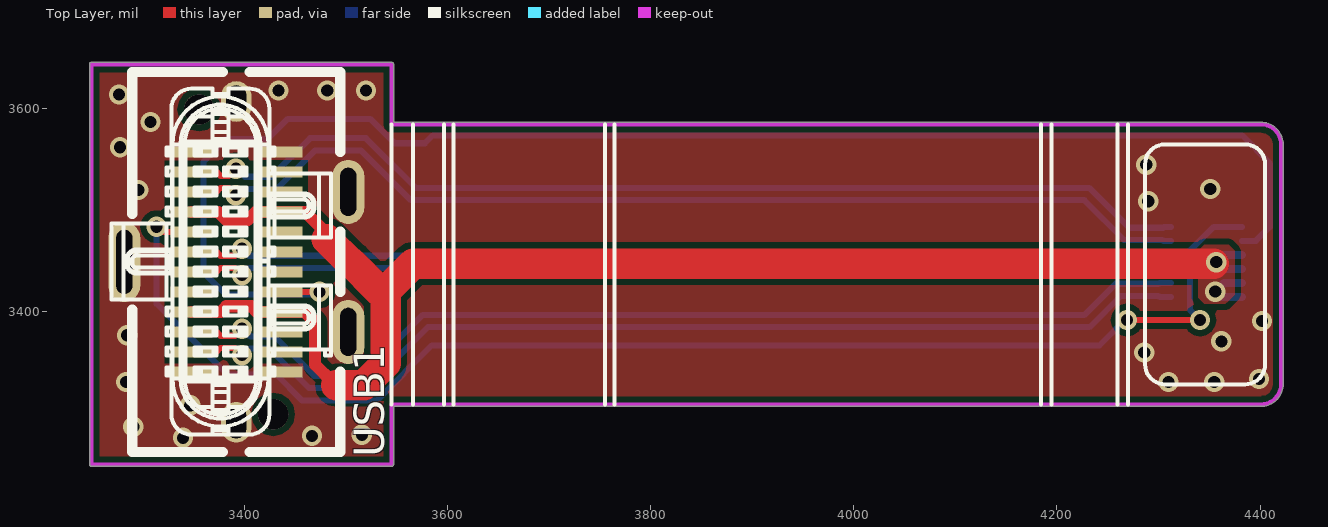
[diagram p0: Top Layer view]
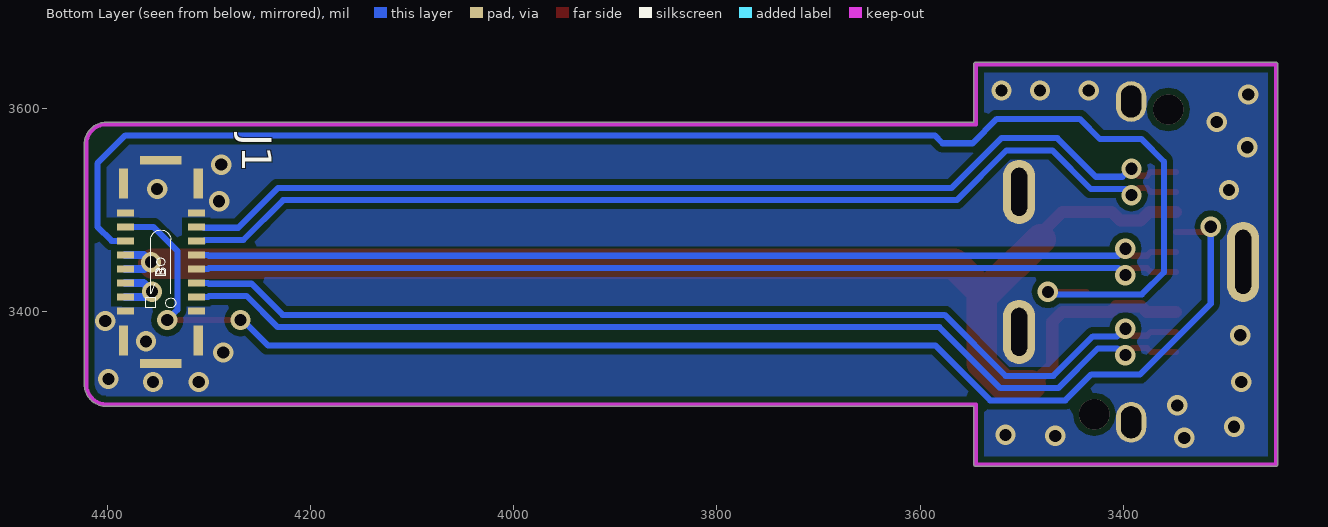
[diagram p1: Bottom Layer view, seen from below]
# Altium PCB MISC89352.pcbdoc
Units mil, origin at the board's own origin, x right, y up, seen from the top; angles counter-clockwise.
Board outline 1174.69 x 397.67 mil, 2 copper layers (Top Layer, Bottom Layer); 2 components, 10 nets, 53 pads, 35 vias.

## Layer stack, top to bottom (the 12.6 mil dielectric is the usual default, probably not edited)
Top Layer: signal copper 1.4
Dielectric: dielectric 12.6, FR-4, Dk 4.8
Bottom Layer: signal copper 1.4

## Board outline
3250,3248.02 cw(c3250,3250) 3248.02,3250 3248.02,3643.7 cw(c3250,3643.7) 3250,3645.68 3545.28,3645.68 cw(c3545.28,3643.7) 3547.26,3643.7 3547.26,3586.63 4401.04,3586.63 cw(c4401.04,3564.96) 4422.7,3564.96 4422.7,3328.74 cw(c4401.04,3328.74) 4401.04,3307.07 3547.26,3307.07 3547.26,3250 cw(c3545.28,3250) 3545.28,3248.02

## Design rules (kind name [scope] priority, off if disabled: settings)
Clearance [All] p1: gap=6
DiffPairsRouting [All] p1: maxlimit=6 minlimit=6 mostfreqgap=6 maxuncoupledlength=500
HoleSize [All] p1: absolutevalues=TRUE maxlimit=500 minlimit=1 maxpercent=80.000 minpercent=20.000
HoleToHoleClearance [All] p1: gap=0 allowstackedmicrovias=TRUE
MinimumSolderMaskSliver [All] p1: minsoldermaskwidth=0
PlaneConnect [All] p1: planeconnectstyle=Direct reliefexpansion=20 reliefentries=4 reliefconductorwidth=10 reliefairgap=10
PolygonConnect [All] p1: connectstyle=Direct reliefconductorwidth=10 reliefentries=4 polygonreliefangle="90 Angle"
RoutingVias [All] p1: holewidth=12 width=20 viastyle="Through Hole" minholewidth=12 minwidth=20 maxholewidth=12 maxwidth=20
SilkToSilkClearance [All] p1: silktosilkclearance=0
SilkscreenOverComponentPads [All] p1: minsilkscreentomaskgap=0
SolderMaskExpansion [All] p1: expansion=4
Width [All] p1: maxlimit=40 minlimit=6 preferedwidth=6 minimp=50.000000 maximp=50.000000 favimp=50.000000
21 further rules are at their usual default settings.

## Classes and differential pairs
differential pair D_D2: +DP2 -DN2
differential pair D_RX1: +RXP1 -RXN1
differential pair D_TX2: +TXP2 -TXN2

## Components (designator, comment, footprint, x,y, rotation, side; value= is the part's Value field where it differs from the comment)
J1 "BK13C06-16DS" BK13C06-16DS_AA 4347.41,3449.24 r90 bottom
USB1 "TYPEC-952-ACP24" USB-C-SMD_TYPEC-952-ACP24 3392.41,3449.24 r270 top locked

## Footprints (in the part's own frame and the unit in brackets; to place one, negate y for a bottom-side part, rotate by r counter-clockwise, add the part's x,y. Pads: shape width x height; smd on the part's side, far side on the other; paste and mask are expansions set on the pad)
BK13C06-16DS_AA [mm]
  rect 0.18x0.425 smd paste+0.102 mask+0.072: 1(-1.225,-0.887) 2(-0.875,-0.887) 3(-0.525,-0.887) 4(-0.175,-0.887) 5(0.175,-0.887) 6(0.525,-0.887) 7(0.875,-0.887) 8(1.225,-0.887) 9(1.225,0.887) 10(0.875,0.887) 11(0.525,0.887) 12(0.175,0.887) 13(-0.175,0.887) 14(-0.525,0.887) 15(-0.875,0.887) 16(-1.225,0.887)
  rect 0.75x0.235 smd paste+0.102 mask+0.05: 17(-1.96,0.932) 18(-1.96,-0.932) 20(1.96,0.932) 21(1.96,-0.932)
  rect 0.215x1.04 smd paste+0.102 mask+0.05: 19(-2.54,0) 22(2.54,0)
  silkscreen extent -1.15,-0.37 0.8,0.38
USB-C-SMD_TYPEC-952-ACP24 [mm]
  round 0.76 hole 0.76 unplated: 0(-3.81,-0.93) 0(3.81,0.92)
  oval 1.6x0.8 hole 0.4 slot 1.2 at 0 deg paste+0 mask+0.05: 1(-1.75,2.8) 2(1.75,2.8)
  oval 1.016x0.762 hole 0.5 slot 0.8 at 0 deg paste+0 mask+0.05: 3(4.01,0) 5(-4.01,0)
  oval 2x0.8 hole 0.4 slot 1.6 at 0 deg paste+0 mask+0.05: 4(0,-2.8)
  rect 0.28x1.06 smd paste-100 mask+0.05: A1(2.75,1.12) A2(2.25,1.12) A3(1.75,1.12) A4(1.25,1.12) A5(0.75,1.12) A6(0.25,1.12) A7(-0.25,1.12) A8(-0.75,1.12) A9(-1.25,1.12) A10(-1.75,1.12) A11(-2.25,1.12) A12(-2.75,1.12) B1(-2.75,-1.12) B2(-2.25,-1.12) B3(-1.75,-1.12) B4(-1.25,-1.12) B5(-0.75,-1.12) B6(-0.25,-1.12) B7(0.25,-1.12) B8(0.75,-1.12) B9(1.25,-1.12) B10(1.75,-1.12) B11(2.25,-1.12) B12(2.75,-1.12)
  silkscreen extent -4.75,-2.6 4.75,2.6

## Part data
J1: "2-0.35V(800)"

## Via types
v1: diameter 20, hole 12, Top Layer to Bottom Layer, 35 vias

## Nets (pads, with @x,y where several pads share a name; then routed paths per layer and width w, separated by ;. In a path a pad name is that pad's centre, name@x,y a point inside that pad or via, vN(x,y) a via of type N, cw(c..) or ccw(c..) an arc to the next point about the centre after c; other vN are vias at no path point)
CC1: J1.11 USB1.A5 | length 1504.4
  Top Layer w6: USB1.A5@3456.71,3419.71 USB1.A5 v1(3474.29,3419.71)
  Bottom Layer w6: v1@3478,3417 3477.76,3417.24 3381.76,3417.24 3360,3439 3360,3548 3382,3570 3423,3570 3443,3590 3524.41,3590 3548.41,3566 3578,3566 ; 3555,3566 3578,3566 ; J1.11 4395.91,3469.91 4409.75,3483.75 4409.75,3546.25 4382.32,3573.68 3585.68,3573.68 3578,3566
CC2: J1.10 USB1.B5 | length 1338.5
  Top Layer w6: v1(3313.92,3483.84) 3318.99,3478.77 USB1.B5 ; v1(4269,3392) v1(4341,3392)
  Bottom Layer w6: v1(3313.92,3483.84) 3314,3483.76 3314,3408 3383.5,3338.5 3431.5,3338.5 3457,3313 3531,3313 3585,3367 4242,3367 v1@4264,3389 ; v1(4341,3392) 4331,3402 4331,3460 4354.69,3483.69 J1.10
DN2: J1.4 USB1.B7 | length 971.9
  Top Layer w6: USB1.B7 3373,3439.4 3376.84,3443.24 3391,3443.24 v1(3398,3436.24)
  Bottom Layer w6: v1(3398,3436.24) 3405,3443.24 4295.76,3443.24 4300.11,3443.24 4301,3442.35 J1.4
DP2: J1.5 USB1.B6 | length 971.9
  Top Layer w6: USB1.B6 3373,3459.08 3376.84,3455.24 3391,3455.24 v1(3398,3462.24)
  Bottom Layer w6: v1(3398,3462.24) 3405,3455.24 4300.11,3455.24 4301,3456.13 J1.5
GND: J1.1 J1.8 J1.9 J1.16 J1.17 J1.18 J1.19 J1.20 J1.21 J1.22 USB1.1 USB1.2 USB1.3 USB1.4 USB1.5 USB1.A1 USB1.A12 USB1.B1 USB1.B12
  other v1: 3340,3276 3467,3278 3516,3279 3291,3287 3347,3308 3284,3331 4310,3331 4355,3331 4399,3334 4286,3360 4362,3371 3285,3377 4402,3391 4290,3509 3296,3520 4351,3521 4288,3545 3278,3562 3308,3587 3277,3614 3434,3618 3482,3618 3520,3618
RXN1: J1.3 USB1.B10 | length 1016.1
  Top Layer w6: USB1.B10 3373,3380.34 3376.84,3376.5 v1@3391,3376.5
  Bottom Layer w6: v1@3398,3384 3405.5,3376.5 3405.87,3376.5 3406.37,3376 3430,3376 3469,3337 3516.03,3337 3576.03,3397 4227.35,3397 4258.03,3427.68 4300.11,3427.68 4301,3428.57 J1.3
  other v1: 3398,3383.5
RXP1: J1.2 USB1.B11 | length 1020.4
  Top Layer w6: USB1.B11 3373,3360.66 3376.84,3364.5 3391,3364.5 v1(3398,3357.5)
  Bottom Layer w6: v1@3402,3360 3406,3364 3425.03,3364 3464.03,3325 3521,3325 3581,3385 4232.32,3385 4263,3415.68 4300.11,3415.68 4301,3414.79 J1.2
TXN2: J1.6 USB1.B3 | length 1013.9
  Top Layer w6: USB1.B3 3373,3518.14 3376.84,3521.98 v1@3385,3521.98
  Bottom Layer w6: v1(3392,3514.98) 3398.02,3521 3432,3521 3470,3559 3515.03,3559 3564.03,3510 4227.03,3510 4266.23,3470.8 4304,3470.8 4304.89,3469.91 J1.6
TXP2: J1.7 USB1.B2 | length 1013.7
  Top Layer w6: USB1.B2 3373,3537.82 3376.84,3533.98 v1@3385,3533.98
  Bottom Layer w6: v1@3393.02,3540.98 3401,3533 3427.03,3533 3465.03,3571 3520,3571 3569,3522 4232,3522 4271.2,3482.8 4304.8,3482.8 4305.69,3483.69 J1.7
  other v1: 3392,3540.98
VBUS: J1.12 J1.13 J1.14 J1.15 USB1.A4 USB1.A9 USB1.B4 USB1.B9 | length 1501
  Top Layer w12: USB1.B9 3377.03,3400.03 3382.5,3405.5 3407.11,3405.5 3412.61,3400 USB1.A4@3437,3400 ; USB1.B4 3374.55,3498.45 3383,3490 3403,3490 3411.45,3498.45 USB1.A9 3460.17,3498.45 3484.31,3474.31 ; USB1.A4 3460.16,3400.03 3470,3390.19 3470,3373 ; 3470,3357.99 3470,3373 ; 3486,3332 3470,3348 3470,3373
  Top Layer w30: 3481.53,3471.53 3505.45,3447.62 3506.38,3447.62 ; 3491,3327.84 3517.86,3327.84 3539.39,3349.37 3539.39,3414.61 3530,3424 ; 3505,3449 3506.38,3447.62 ; v1@4354.62,3447.62 3566.62,3447.62 3543,3424 3530,3424 ; 3506.38,3447.62 3530,3424
  Bottom Layer w8: v1(4356,3420) 4357,3421 4364.57,3428.57 J1.14 ; v1@4359,3447 4363.65,3442.35 J1.13 ; v1@4360,3418 4363.21,3414.79 J1.15 ; 4364.13,3456.13 J1.12
  other v1: 4357,3449
pads on no net: USB1.0 USB1.A2 USB1.A3 USB1.A6 USB1.A7 USB1.A8 USB1.A10 USB1.A11 USB1.B8

## Polygon pours and split planes (outlines as drawn)
VBUS on Top Layer "Bottom Layer-No Net" (solid, remove dead copper, pour order 1000): 4339,3447 4339,3429 4339,3414 4341,3412 4345,3408 4350,3408 4366,3408 4368,3410 4373,3415 4375,3417 4375,3455 4375,3460 4371,3464 4369,3466 4363,3466 4345,3466 4341,3462 4339,3460 4339,3447
GND on Top Layer "Bottom Layer-No Net" (solid, remove dead copper, pour order 1001): 3139,3659.8 3139,3236.8 3163,3212.8 3198,3177.8 3312,3177.8 4357,3177.8 4427,3247.8 4435,3255.8 4435,3285.8 4435,3644.8 4364,3715.8 4333,3746.8 4312,3746.8 3220,3746.8 3136,3662.8
GND on Bottom Layer "Bottom Layer-No Net" (solid, remove dead copper, pour order 1002): 3189.37,3607.18 3191.37,3605.18 3191.37,3196.18 4464.37,3196.18 4477.37,3209.18 4482.37,3214.18 4482.37,3242.18 4482.37,3601.18 4423.37,3660.18 4363.37,3720.18 3848.37,3720.18 3254.37,3720.18 3211.37,3677.18 3194.37,3660.18 3194.37,3612.18

## Keep-outs
Board Outline Layer:
  lines w3.94: 3566.39,3584.65 4184.42,3584.65 ; 3596.7,3584.65 3545.28,3584.65 3545.28,3643.7 3250,3643.7 3250,3250 3545.28,3250 3545.28,3309.06 3755.08,3309.06 ; 3606.32,3309.06 4401.04,3309.06 ccw(c4401.04,3328.74) 4420.72,3328.74 4420.72,3564.96 ccw(c4401.04,3564.96) 4401.04,3584.65 4194.98,3584.65 ; 3764.7,3584.65 4259.7,3584.65

## Silkscreen, mask and mechanical layers (free items; w line width, h text height)
Top Silkscreen Layer:
  drawing of 481 lines, arcs and shapes, not listed